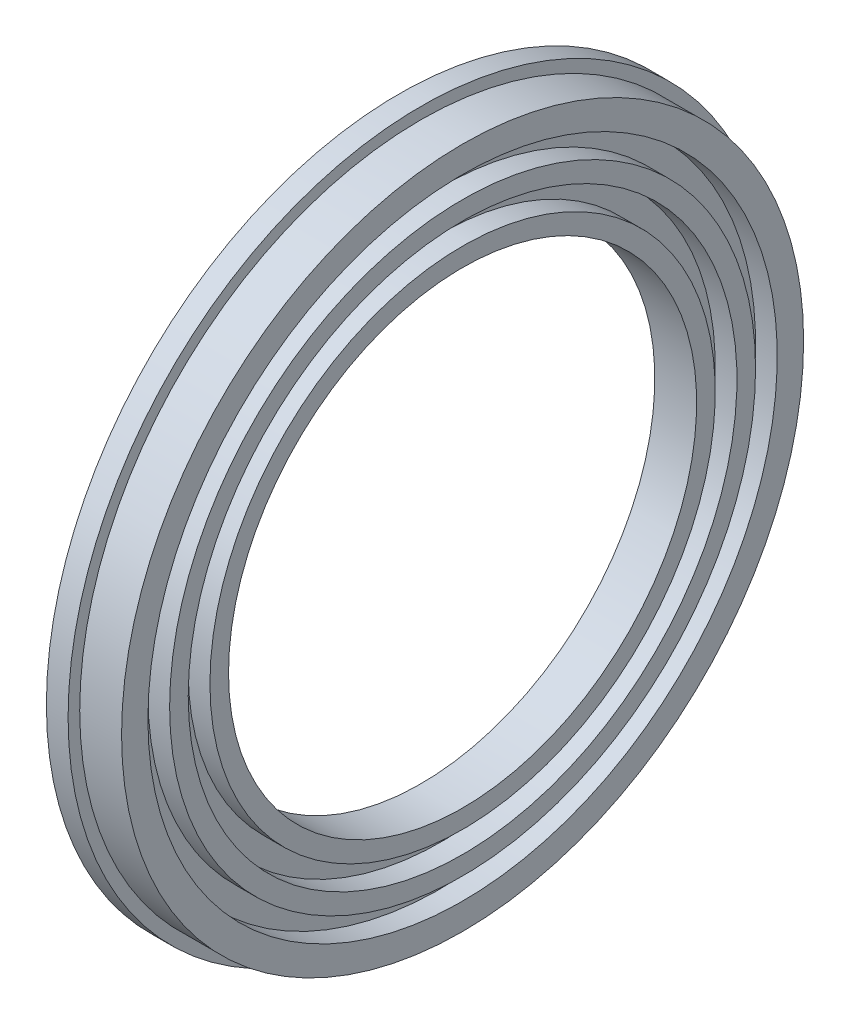
SolidWorks part; units mm, degrees
material "灰铸铁 HT150 "
ref_plane "Front Plane" through (0, 0, 0) normal (0, 0, 1) x (1, 0, 0)
ref_plane "Top Plane" through (0, 0, 0) normal (0, 1, 0) x (1, 0, 0)
ref_plane "Right Plane" through (0, 0, 0) normal (1, 0, 0) x (0, 0, -1)
sketch "Sketch1" plane through (0, 0, 0) normal (0, 1, 0) x (1, 0, 0)
  line L0 (0, 0) -> (170.742, 0) construction
  line L1 (0, 200) -> (0, 227.5)
  line L2 (0, 227.5) -> (14, 227.5)
  line L3 (14, 227.5) -> (14, 220)
  line L4 (14, 220) -> (41, 220)
  line L5 (41, 220) -> (41, 203)
  line L6 (41, 151) -> (14, 151)
  line L7 (14, 151) -> (14, 200)
  line L8 (14, 200) -> (0, 200)
  line L13 (41, 189) -> (41, 177)
  line L14 (41, 203) -> (27, 203)
  line L15 (41, 189) -> (27, 189)
  line L16 (27, 203) -> (27, 189)
  line L17 (41, 163) -> (41, 151)
  line L18 (41, 177) -> (27, 177)
  line L19 (41, 163) -> (27, 163)
  line L20 (27, 177) -> (27, 163)
  dimension "D1" = 151
  dimension "D2" = 200
  dimension "D3" = 227.5
  dimension "D4" = 14
  dimension "D5" = 41
  dimension "D6" = 220
  dimension "D7" = 203
  dimension "D8" = 14
  dimension "D9" = 14
  dimension "D10" = 163
  dimension "D11" = 177
  dimension "D12" = 189
revolve "Revolve1" add sketch "Sketch1" angle 360 about L0
fillet "Fillet1" radius 10 1 edges at (14, 0, 200)
